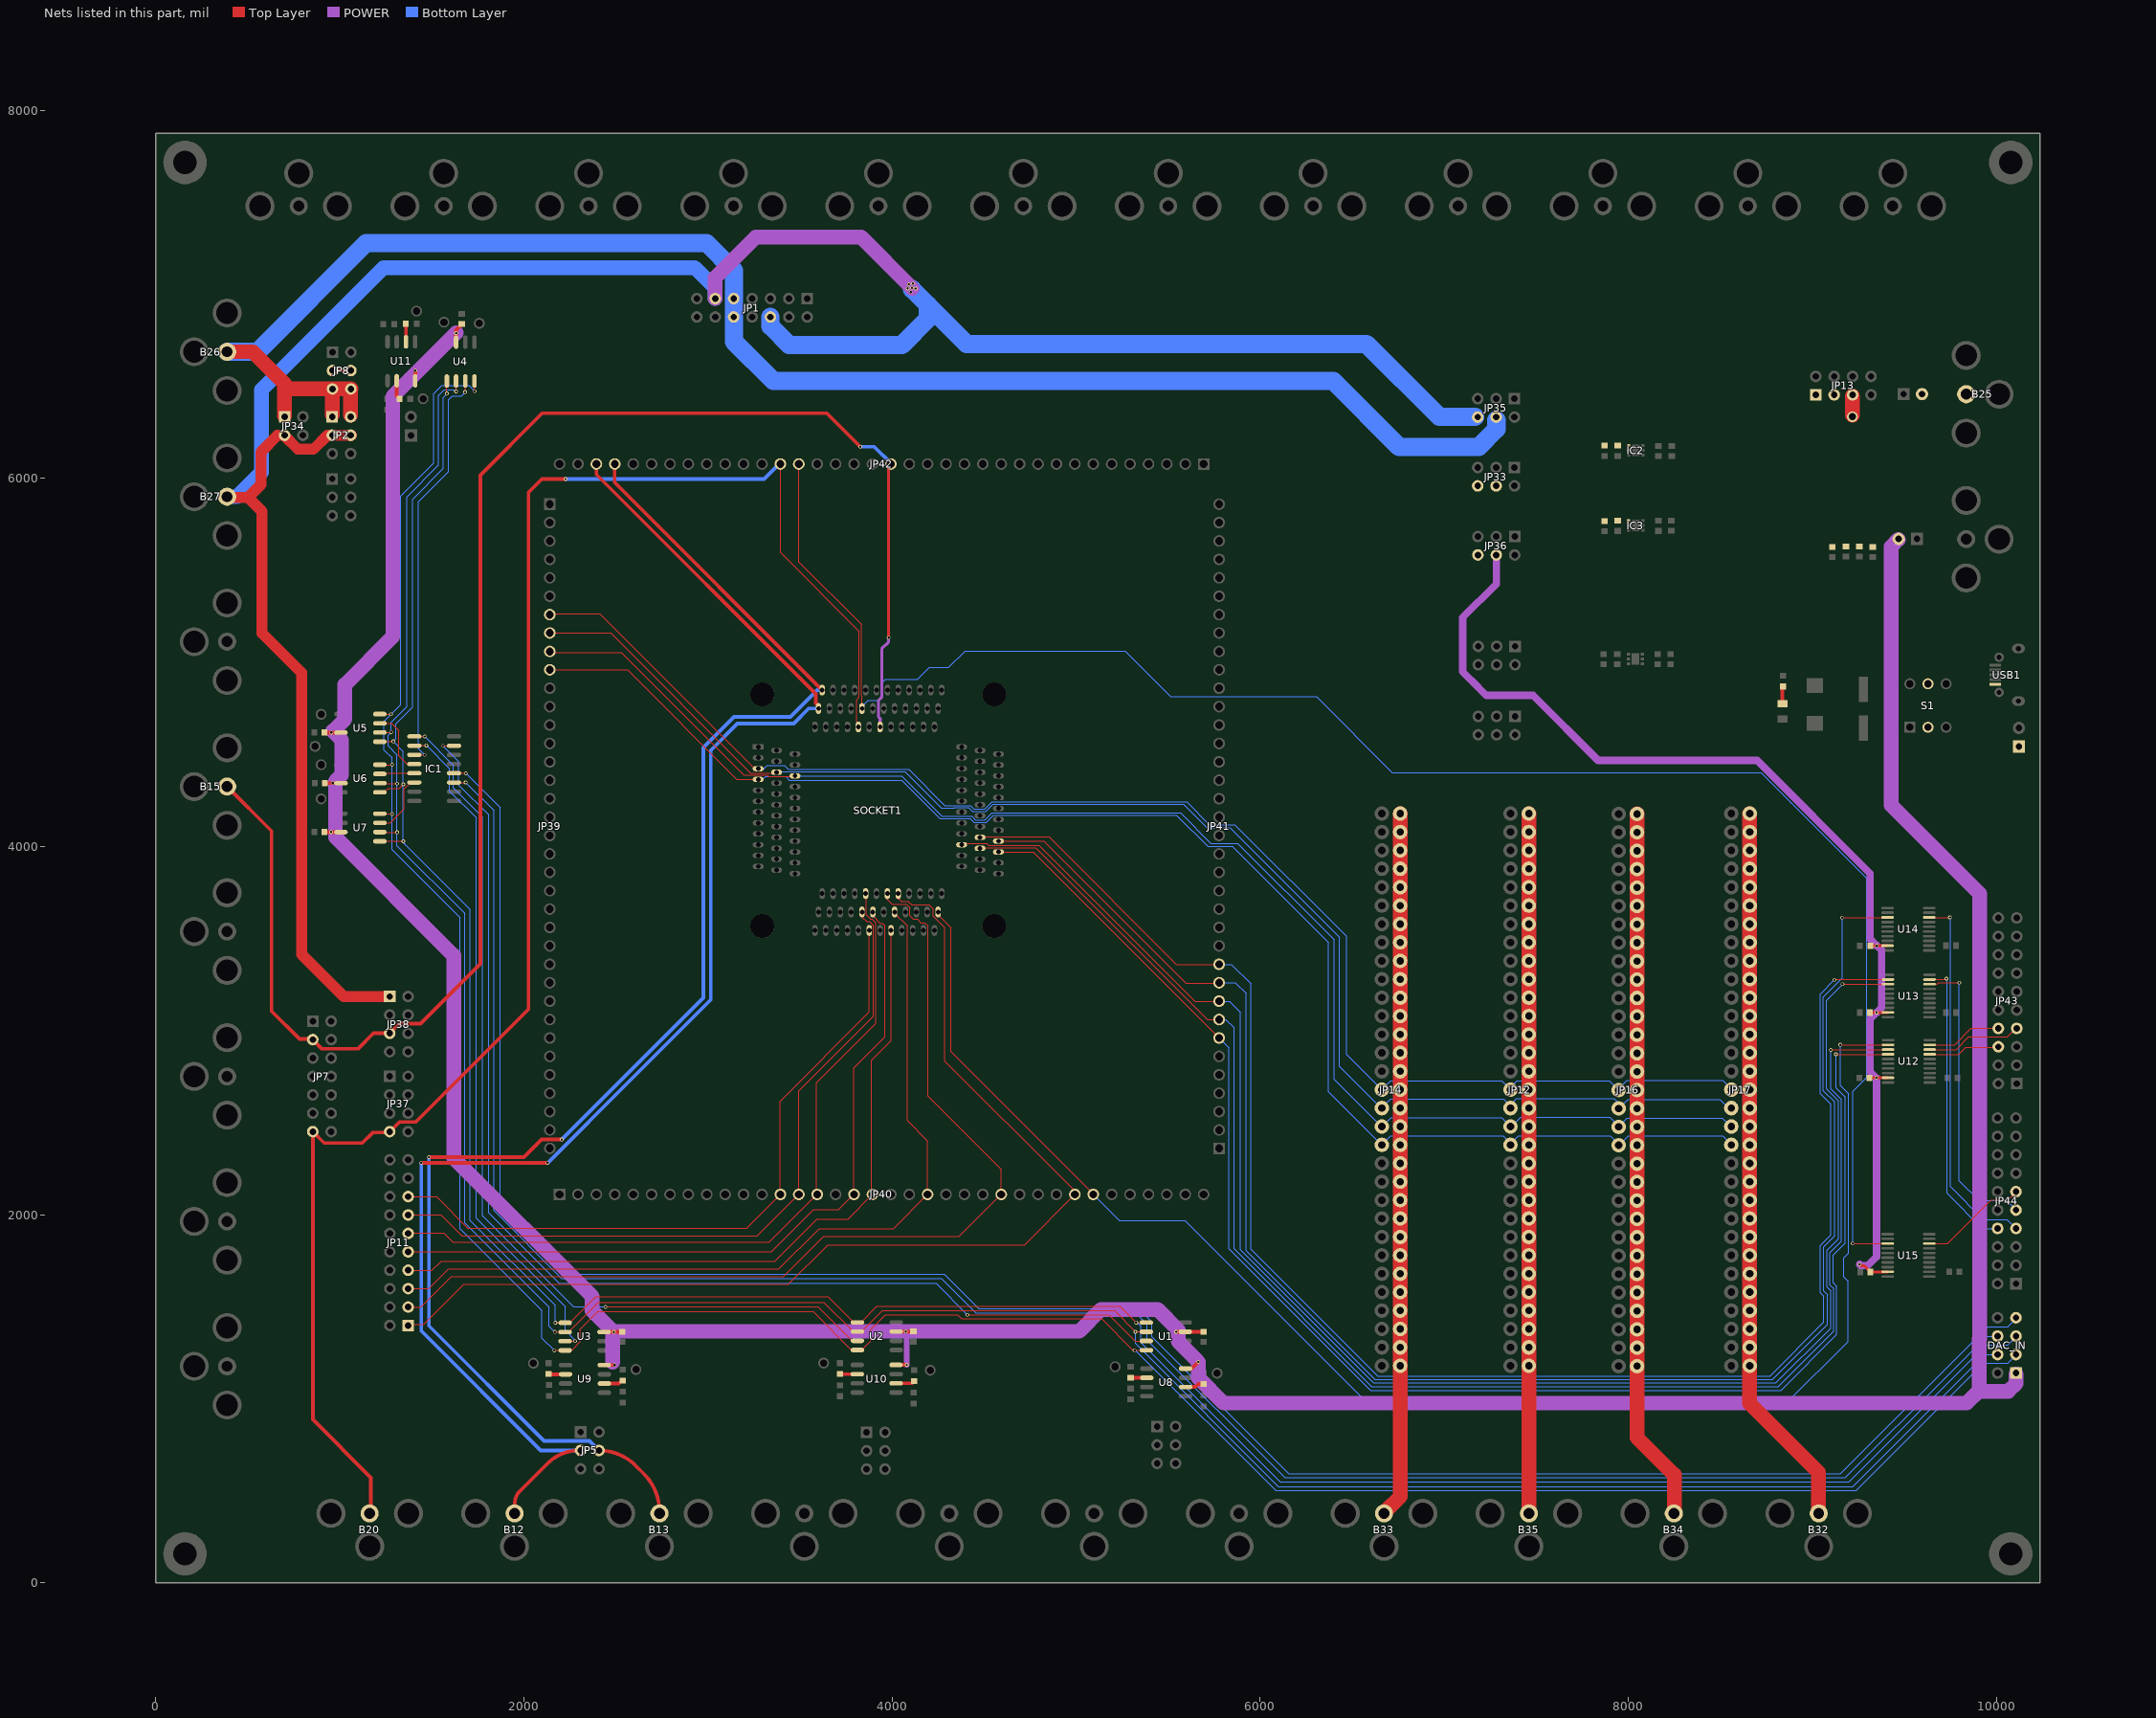
[diagram p0: the nets of this part, all layers, seen from the top]
# Altium PCB MISC62794.PcbDoc (part 4 of 7)
Units mil, origin at the board's own origin, x right, y up, seen from the top; angles counter-clockwise.
Board outline 10236.22 x 7874.02 mil, 4 copper layers (Top Layer, GND, POWER, Bottom Layer); 158 components, 185 nets, 1211 pads, 1759 vias.

## Via types
v1: diameter 20, hole 12, Top Layer to Bottom Layer, 1759 vias

## Nets (pads, with @x,y where several pads share a name; then routed paths per layer and width w, separated by ;. In a path a pad name is that pad's centre, name@x,y a point inside that pad or via, vN(x,y) a via of type N, cw(c..) or ccw(c..) an arc to the next point about the centre after c; other vN are vias at no path point) (continued)
IREF: B15.1 JP7.3 JP38.5 JP42.18 SOCKET1.126 | length 9370.4
  Top Layer w16: v1(3981,5135) 3981,6057 JP42.18@3993,6069
  Top Layer w20: B15.1@386.77,4325.69 628,4084.47 628,3106 780,2954 JP7.3@854,2954 ; JP7.3@852,2951 902,2901 1097,2901 1182,2986 ; 1222.43,2986 1182,2986 ; JP38.5@1258,2986 1182,2986 ; JP38.5@1269.93,2985.09 1321.83,3037 1437,3037 1762,3362 1762,5790 ; 1762,5819 1762,5790 ; v1(3827,6172) 3645,6354 2098,6354 1762,6018 1762,5790
  POWER w16: SOCKET1.126@3934.84,4649.77 3934.84,4695.16 3926.16,4703.84 3926.16,4793.16 3943.53,4810.53 3943.53,5074.53 3981,5112 v1(3981,5135)
  Bottom Layer w20: v1(3827,6172) 3903,6172 JP42.18@3988,6087
NetB25_1: B25.1 JP30.2
NetB32_1: B32.1 JP17.2 JP17.4 JP17.6 JP17.8 JP17.10 JP17.12 JP17.14 JP17.16 JP17.18 JP17.20 JP17.22 JP17.24 JP17.26 JP17.28 JP17.30 JP17.32 JP17.34 JP17.36 JP17.38 JP17.40 JP17.42 JP17.44 JP17.46 JP17.48 JP17.50 JP17.52 JP17.54 JP17.56 JP17.58 JP17.60 JP17.62 | length 3955.5
  Top Layer w80: JP17.62@8660,4179 JP17.60@8660,4079 JP17.58@8660,3979 JP17.56@8660,3879 JP17.54@8660,3779 JP17.52@8660,3679 JP17.50@8660,3579 JP17.48@8660,3479 JP17.46@8660,3379 JP17.44@8660,3279 JP17.42@8660,3179 JP17.40@8660,3079 JP17.38@8660,2979 JP17.36@8660,2879 JP17.34@8660,2779 JP17.32@8660,2679 JP17.30@8660,2579 JP17.28@8660,2479 JP17.26@8660,2379 JP17.24@8660,2279 JP17.22@8660,2179 JP17.20@8660,2079 JP17.18@8660,1979 JP17.16@8660,1879 JP17.14@8660,1779 JP17.12@8660,1679 JP17.10@8660,1579 JP17.8@8660,1479 JP17.6@8660,1379 JP17.4@8660,1279 JP17.2@8660,1179 8660,974 9033,601 B32.1@9033,378
NetB33_1: B33.1 JP14.2 JP14.4 JP14.6 JP14.8 JP14.10 JP14.12 JP14.14 JP14.16 JP14.18 JP14.20 JP14.22 JP14.24 JP14.26 JP14.28 JP14.30 JP14.32 JP14.34 JP14.36 JP14.38 JP14.40 JP14.42 JP14.44 JP14.46 JP14.48 JP14.50 JP14.52 JP14.54 JP14.56 JP14.58 JP14.60 JP14.62 | length 3836.9
  Top Layer w80: B33.1@6672.81,377.15 B33.1@6672.81,382 ; B33.1@6675,382 6762,469 6762,907 6762,1279 6762,1679 6762,2179 6762,2679 6762,3179 6762,3379 6762,3579 6762,3979 JP14.62@6762,4178
NetB34_1: B34.1 JP16.2 JP16.4 JP16.6 JP16.8 JP16.10 JP16.12 JP16.14 JP16.16 JP16.18 JP16.20 JP16.22 JP16.24 JP16.26 JP16.28 JP16.30 JP16.32 JP16.34 JP16.36 JP16.38 JP16.40 JP16.42 JP16.44 JP16.46 JP16.48 JP16.50 JP16.52 JP16.54 JP16.56 JP16.58 JP16.60 JP16.62 | length 3868.7
  Top Layer w80: JP16.62@8048,4177.02 JP16.60@8048,4077.02 JP16.58@8048,3977.02 JP16.56@8048,3877.02 JP16.54@8048,3777.02 JP16.52@8048,3677.02 JP16.50@8048,3577.02 JP16.48@8048,3477.02 JP16.46@8048,3377.02 JP16.44@8048,3277.02 JP16.42@8048,3177.02 JP16.40@8048,3077.02 JP16.38@8048,2977.02 JP16.36@8048,2877.02 JP16.34@8048,2777.02 JP16.32@8048,2677.02 JP16.30@8048,2577.02 JP16.28@8048,2477.02 JP16.26@8048,2377.02 JP16.24@8048,2277.02 JP16.22@8048,2177.02 JP16.20@8048,2077.02 JP16.18@8048,1977.02 JP16.16@8048,1877.02 JP16.14@8048,1777.02 JP16.12@8048,1677.02 JP16.10@8048,1577.02 JP16.8@8048,1477.02 JP16.6@8048,1377.02 JP16.4@8048,1277.02 JP16.2@8048,1177.02 8048,789 8250,587 B34.1@8250,392
NetB35_1: B35.1 JP12.2 JP12.4 JP12.6 JP12.8 JP12.10 JP12.12 JP12.14 JP12.16 JP12.18 JP12.20 JP12.22 JP12.24 JP12.26 JP12.28 JP12.30 JP12.32 JP12.34 JP12.36 JP12.38 JP12.40 JP12.42 JP12.44 JP12.46 JP12.48 JP12.50 JP12.52 JP12.54 JP12.56 JP12.58 JP12.60 JP12.62 | length 3786
  Top Layer w80: B35.1@7460,393 JP12.2@7460,1179 JP12.4@7460,1279 JP12.6@7460,1379 JP12.8@7460,1479 JP12.10@7460,1579 JP12.12@7460,1679 JP12.14@7460,1779 JP12.16@7460,1879 JP12.18@7460,1979 JP12.20@7460,2079 JP12.22@7460,2179 JP12.24@7460,2279 JP12.26@7460,2379 JP12.28@7460,2479 JP12.30@7460,2579 JP12.32@7460,2679 JP12.34@7460,2779 JP12.36@7460,2879 JP12.38@7460,2979 JP12.40@7460,3079 JP12.42@7460,3179 JP12.44@7460,3279 JP12.46@7460,3379 JP12.48@7460,3479 JP12.50@7460,3579 JP12.52@7460,3679 JP12.54@7460,3779 JP12.56@7460,3879 JP12.58@7460,3979 JP12.60@7460,4079 JP12.62@7460,4179
NetJP13_5: JP13.5 TP15.1 | length 104
  Top Layer w80: TP15.1@9218,6343 JP13.5@9218,6447
NetJP32_1: JP32.1 S1.2
NetLED_BLUE_2: LED_BLUE.2 R20.1 | length 82.7
  Top Layer w20: LED_BLUE.2@8838,4775.33 R20.1@8838,4858
NetR1_1: R1.1 U8.2 | length 80.8
  Top Layer w20: R1.1@5302.67,1113.67 U8.2@5383.51,1113.67
NetR3_2: R3.2 U8.6 | length 99
  Top Layer w20: U8.6@5594.73,1063.67 5648.67,1063.67 5665,1080 R3.2@5687,1080
NetR5_1: R5.1 U10.2 | length 90.2
  Top Layer w20: R5.1@3720.33,1133.67 U10.2@3810.51,1133.67
NetR7_2: R7.2 U10.6 | length 102.8
  Top Layer w20: U10.6@4021.73,1083.67 4105.67,1083.67 R7.2@4119,1097
NetR9_1: R9.1 U9.2 | length 88.2
  Top Layer w20: R9.1@2137.33,1132.67 U9.2@2225.51,1132.67
NetR11_2: R11.2 U9.6 | length 101
  Top Layer w20: U9.6@2436.73,1082.67 2514.67,1082.67 R11.2@2531,1099
NetR13_1: R13.1 U11.2 | length 86.3
  Top Layer w20: U11.2@1358.29,6741.99 R13.1@1358.29,6828.29
NetR15_2: R15.2 U11.6 | length 103.9
  Top Layer w20: U11.6@1308.29,6530.77 1308.29,6447.71 R15.2@1323,6433
NetS1_5: S1.5 USB1.1
OEN: JP41.9 SOCKET1.81 U13.13 | length 9034.7
  Top Layer w6: SOCKET1.81@4385,4009 4393,4017 4515,4017 4525.68,4006.32 4798.68,4006.32 5644.98,3160.02 JP41.9@5777,3160.02 ; v1@9168.01,3251.99 U13.13@9410.97,3251.99
  Bottom Layer w6: JP41.9@5777,3160.02 5831.98,3160.02 5893,3099 5893,1976 ; 5893,1960 5893,1976 ; v1@9163,3250 9078,3165 9078,2893 9078,2683 9142,2619 9142,1869 9081,1808 9081,1606 9101,1586 9101,1384 8803,1086 6616,1086 5893,1809 5893,1976 ; v1@9164,3250 v1(9164,3252)
OEN_MCU: JP44.9 U13.8 | length 1615.6
  Top Layer w6: U13.8@9637.03,3251.99 9678.99,3251.99 9687,3260 v1(9799,3260)
  Bottom Layer w6: v1@9804,3259 9799,3254 9799,2185 9907,2077 10055.01,2077 JP44.9@10107,2025.01
OUT<0>: JP11.1 JP40.29 SOCKET1.60 | length 6042.2
  Top Layer w6: JP11.1@1384,1404 1455,1404 1673,1622 3437,1622 3651,1836 4718.98,1836 JP40.29@4993,2110.02 ; SOCKET1.60@4033.27,3744.26 4033.27,3718.73 4049,3703 4086,3703 4106.21,3682.79 4200.43,3682.79 4223,3660.22 4223,3622 4287,3558 4287,2835 4947,2175 ; 4970,2152 4947,2175 ; JP40.29@5004,2115 5004,2118 4947,2175
OUT<1>: JP11.5 JP40.21 SOCKET1.59 | length 4653
  Top Layer w6: JP11.5@1370.64,1598.09 1482.09,1598.09 1589,1705 3384,1705 3604,1925 4007.98,1925 JP40.21@4193,2110.02 ; SOCKET1.59@4013.58,3644.26 4013.58,3638.42 4082,3570 4082,2511 4193,2400 4193,2186 ; JP40.21@4193,2124 4193,2186 ; 4193,2162 4193,2186
OUT<2>: JP11.7 JP40.18 SOCKET1.58 | length 4134.8
  Top Layer w6: JP11.7@1388,1697 1500,1697 1551,1748 3363,1748 3592,1977 3759.98,1977 JP40.18@3893,2110.02 ; JP40.18@3889,2129 3889,2840 3993.9,2944.9 SOCKET1.58@3993.9,3544.26
OUT<3>: JP11.3 JP40.25 SOCKET1.57 | length 5460.1
  Top Layer w6: JP11.3@1370.64,1498.09 1440.09,1498.09 1605,1663 3410,1663 3628,1881 4363.98,1881 JP40.25@4593,2110.02 ; SOCKET1.57@3974.21,3744.26 3974.21,3712.79 3999.95,3687.05 4078.05,3687.05 4096.01,3669.1 4096.01,3623.99 4115,3605 4138,3605 4157,3586 4177.53,3586 4194.43,3569.1 4194.43,2644.57 4594,2245 4594,2204 ; JP40.25@4594,2127 4594,2204 ; 4594,2165 4594,2204
OUT<4>: JP11.9 JP40.17 SOCKET1.53 | length 4217.7
  Top Layer w6: JP11.9@1374,1799 1473,1799 ; 1421,1799 1473,1799 ; JP40.17@3793,2110.02 3709.98,2027 3573,2027 3345,1799 1473,1799 ; JP40.17@3793,2127 3793,2189 ; 3793,2180 3793,2189 ; SOCKET1.53@3895.47,3636.53 SOCKET1.53@3895.47,3644.26 ; SOCKET1.53@3898,3624 3898,3621 3936.21,3582.79 3949.21,3582.79 3962,3570 3962,2967 3793,2798 3793,2189
OUT<5>: JP11.15 JP40.13 SOCKET1.52 | length 3798.7
  Top Layer w6: JP11.15@1380,2098 1524,2098 1695,1927 3209.98,1927 JP40.13@3393,2110.02 ; JP40.13@3391,2124 3391,2180 ; 3391,2162 3391,2180 ; SOCKET1.52@3875.79,3544.26 3875.79,3100.79 3391,2616 3391,2180
OUT<6>: JP11.11 JP40.15 SOCKET1.51 | length 4130.2
  Top Layer w6: JP11.11@1375,1900 1564,1900 1614,1850 3332.98,1850 JP40.15@3593,2110.02 ; JP40.15@3590,2139 3590,2192 ; 3590,2174 3590,2192 ; SOCKET1.51@3856.1,3744.26 3859.79,3740.57 3859.79,3629.21 3883.27,3605.73 3891.27,3605.73 3911.16,3585.84 3911.16,3038.16 3590,2717 3590,2192
OUT<7>: JP11.13 JP40.14 SOCKET1.50 | length 4007.3
  Top Layer w6: JP11.13@1375,2000 1548,2000 1663,1885 3267.98,1885 JP40.14@3493,2110.02 ; JP40.14@3493,2120 3493,2202 ; 3493,2182 3493,2202 ; SOCKET1.50@3836.42,3644.26 3836.42,3616.58 3861,3592 3878,3592 3899.16,3570.84 3899.16,3079.16 3493,2673 3493,2202
RCLK: DAC_IN.7 IC1.12 | length 11719.8
  Top Layer w6: IC1.12@1619.33,4398.08 v1(1683.08,4398.08)
  Bottom Layer w6: v1(1683.08,4398.08) 1870,4211.16 1870,2024 2218,1676 4284,1676 4470,1490 5341,1490 5413,1418 5413,1335 6155,593 9154,593 9953,1392 10064,1392 DAC_IN.7@10091,1419
READ_EN: JP41.11 SOCKET1.83 U13.12 | length 8978.2
  Top Layer w6: SOCKET1.83@4498.94,4053.06 4851.94,4053.06 5544.98,3360.02 JP41.11@5777,3360.02 ; v1@9124,3274 9127.58,3277.58 U13.12@9410.97,3277.58
  Bottom Layer w6: JP41.11@5777,3360.02 5842.98,3360.02 5949,3254 5949,1813 6639,1123 8770,1123 9063,1416 9063,1558 9045,1576 9045,1834 9101,1890 9101,2599 9043,2657 9043,3199 v1@9120,3276
  other v1: 9121,3276
READ_EN_MCU: JP44.8 U13.9 | length 1612.5
  Top Layer w6: U13.9@9637.03,3277.58 9724.58,3277.58 v1(9729,3282)
  Bottom Layer w6: v1@9732,3280 9732,2115 9921.99,1925.01 JP44.8@10007,1925.01
SCLK: DAC_IN.6 IC1.11 | length 11592.8
  Top Layer w6: IC1.11@1619.33,4348.08 v1(1682.92,4348.08)
  Bottom Layer w6: v1(1682.92,4348.08) 1836,4195 1836,2022 2204,1654 4269,1654 4455.5,1467.5 5323.5,1467.5 5387,1404 5387,1318 6134,571 9179,571 9742,1134 ; 9745,1137 9742,1134 ; 9966.5,1340 9958,1340 ; DAC_IN.6@9993,1340 9958,1340 ; 9742,1134 9948,1340 9958,1340
SPI_CLK: DAC_IN.5 U1.1 U2.1 U3.1 U4.1 U5.1 U6.1 U7.1 | length 14765.3
  Top Layer w6: U7.1@1216.15,4028.46 v1(1344.54,4028.46) ; U5.1@1235,4571 v1(1290,4571) ; U6.1@1247,4301 1262,4316 1322,4316 v1(1344,4338) ; v1(1580.71,6461.29) U4.1@1580.71,6529.01 ; v1(2170.33,1412.67) U3.1@2223.51,1412.67 ; U3.1@2245,1410 2390,1555 3652,1555 3792.33,1414.67 U2.1@3811.51,1414.67 ; U2.1@3835,1420 3918,1503 5237.34,1503 v1(5326.67,1413.67) U1.1@5381.51,1413.67
  Bottom Layer w6: 1352,4013 1356,4009 ; v1@1578.5,6457.5 v1@1581,6460 ; v1@1579,6457 1562,6440 1562,6054 1395,5887 1395,4757 1305,4667 1305,4586 v1(1290,4571) 1344,4517 v1(1344,4338) 1344,4021 1356,4009 ; v1(2170.33,1412.67) 2170.33,1506.67 1708,1969 1708,3657 1356,4009 ; v1(5326.67,1413.67) 5330.33,1413.67 5351,1393 5351,1306 6109,548 9200,548 9777,1125 ; 9779,1127 9777,1125 ; DAC_IN.5@10099,1329 10062,1292 9944,1292 9777,1125
SPI_CS1: IC1.15 U1.3 | length 6545.5
  Top Layer w6: v1(1559,4547) 1599,4547 IC1.15@1600,4546 ; v1(4409,1456) 4409,1457 5177,1457 5320.33,1313.67 U1.3@5381.51,1313.67
  Bottom Layer w6: v1(1559,4547) 1645,4461 1645,4335 1807,4173 1807,2010 2190,1627 4238,1627 v1(4409,1456)
SPI_CS2: IC1.1 U2.3 | length 5080.4
  Top Layer w6: IC1.1@1434,4599 1435,4598 v1(1460,4598) ; v1(2443,1499) 3597,1499 3781.33,1314.67 U2.3@3811.51,1314.67
  Bottom Layer w6: v1(1460,4598) 1617,4441 1617,4319 1775,4161 1775,1993 2268,1500 v1@2442,1500 ; v1(2443,1499) v1@2442,1500 ; v1@2443,1500 v1@2442,1500
SPI_CS3: IC1.2 U3.3 | length 3676.6
  Top Layer w6: IC1.2@1421,4552 1424,4549 v1(1469,4549) ; U3.3@2223.51,1312.67 v1(2277.33,1312.67)
  Bottom Layer w6: v1(1469,4549) 1596,4422 1596,4300 1740,4156 1740,1982 2223,1499 2223,1372 v1@2277.33,1317.67 ; v1(2277.33,1312.67) v1@2277.33,1317.67 ; v1@2279,1316 v1@2277.33,1317.67
SPI_CS4: IC1.3 U4.3 | length 2220.9
  Top Layer w6: IC1.3@1403.94,4498.08 v1(1459.92,4498.08) ; v1(1680,6469) U4.3@1680,6508
  Bottom Layer w6: v1(1459.92,4498.08) 1426,4532 1426,5874 1590,6038 1590,6293 ; 1590,6300 1590,6293 ; v1@1677,6466 v1(1680,6469) ; v1@1678,6465 1661,6448 1611,6448 1590,6427 1590,6379 1590,6376 1590,6293
SPI_CS5: IC1.4 U5.3 | length 339.3
  Top Layer w6: U5.3@1238,4670 1280,4670 1319,4631 1319,4492 1362.92,4448.08 IC1.4@1403.94,4448.08
SPI_CS6: IC1.5 U6.3 | length 153.9
  Top Layer w6: U6.3@1250.08,4398.08 IC1.5@1403.94,4398.08
SPI_CS7: IC1.6 U7.3 | length 342
  Top Layer w6: U7.3@1216.15,4128.46 1272.46,4128.46 1348,4204 1348,4312 1384.08,4348.08 IC1.6@1403.94,4348.08
SPI_MISO: DAC_IN.3 U1.4 U2.4 U3.4 U4.4 U5.4 U6.4 U7.4 | length 15066.1
  Top Layer w6: U7.4@1237,4178 1238,4177 v1(1283,4177) ; U5.4@1241,4718 v1@1276,4718 ; U6.4@1243,4446 1245,4444 v1(1283,4444) ; v1(1731,6474) U4.4@1731,6503 ; v1(2164.67,1262.67) U3.4@2223.51,1262.67 ; U3.4@2236,1265 2262,1265 2306,1309 2306,1378 2402,1474 3570,1474 3779.33,1264.67 U2.4@3811.51,1264.67 ; U2.4@3836,1267 3837,1267 3884,1314 3884,1375 3964,1455 4355,1455 4376,1434 5138,1434 5308.33,1263.67 v1(5317.67,1263.67) U1.4@5381.51,1263.67
  Bottom Layer w6: v1(1731,6474) 1701,6504 1554,6504 1510,6460 1510,6084 1330,5904 1330,4772 v1(1277,4719) 1239,4681 1239,4525 1283,4481 v1(1283,4444) v1(1283,4177) 1283,3984 1652,3615 1652,1925 2098,1479 2098,1329.34 v1(2164.67,1262.67) ; v1@5321.33,1263.67 6084,501 9239,501 9930,1192 10062,1192 DAC_IN.3@10091,1221
SPI_MOSI: DAC_IN.4 U1.2 U2.2 U3.2 U4.2 U5.2 U6.2 U7.2 | length 14708.1
  Top Layer w6: U5.2@1216.15,4619.46 1279.46,4619.46 v1@1281,4621 ; U7.2@1233,4079 1235,4077 v1(1310,4077) ; U6.2@1235,4342 v1(1310,4342) ; U4.2@1630,6501 1631,6500 v1(1631,6472) ; v1(2166.67,1362.67) U3.2@2223.51,1362.67 2241.67,1362.67 2403,1524 3629,1524 U2.2@3789,1364 ; U2.2@3811.51,1364.67 3833.67,1364.67 3947,1478 5208,1478 v1@5318,1368 ; v1(5322.33,1363.67) U1.2@5381.51,1363.67
  Bottom Layer w6: 1536,6296 1536,6291 ; v1@1627,6474 1619,6482 1567,6482 1536,6451 1536,6291 ; v1@1628,6475 v1(1631,6472) ; v1(2166.67,1362.67) 2136,1393.34 2136,1497 1678,1955 1678,3637 1310,4005 v1(1310,4077) v1(1310,4342) 1310,4497 1261,4546 1261,4605 v1(1278,4622) 1278,4675 1363,4760 1363,5899 1536,6072 1536,6291 ; v1(5322.33,1363.67) 5322.33,1299.67 6099,523 9221,523 9804,1106 ; 9809,1111 9804,1106 ; DAC_IN.4@9986,1239 9937,1239 9804,1106
STATE<0>: JP41.7 SOCKET1.79 U12.14 | length 8514.4
  Top Layer w6: SOCKET1.79@4580,3969 4768.02,3969 JP41.7@5777,2960.02 ; v1(9128.6,2871.4) U12.14@9411.97,2871.4
  Bottom Layer w6: JP41.7@5777,2960.02 5830,2907.02 5830,2096 ; 5830,1970 5830,2096 ; v1@9129,2869 9129,2689 9134,2684 9178,2640 9178,1847 9113,1782 9113,1629 9133,1609 9133,1348 8831,1046 6599,1046 5830,1815 5830,2096
STATE<0>_MCU: JP43.6 U12.7 | length 376
  Top Layer w6: U12.7@9638.03,2871.4 9794.4,2871.4 9833,2910 JP43.6@9998,2910
STATE<1>: JP41.8 SOCKET1.80 U12.13 | length 8566.2
  Top Layer w6: SOCKET1.80@4477.76,3990.32 4481.44,3994.01 4778.99,3994.01 5714,3059 JP41.8@5766,3059 ; v1@9102,2900 9105.01,2896.99 U12.13@9411.97,2896.99
  Bottom Layer w6: JP41.8@5777,3060.02 5812.98,3060.02 5858,3015 5858,1814 6605,1067 8816,1067 9117,1368 9117,1598 9097,1618 9097,1794 9158,1855 9158,2627 9101,2684 v1(9101,2895)
STATE<1>_MCU: JP43.7 U12.8 | length 504.3
  Top Layer w6: U12.8@9638.03,2896.99 9781.99,2896.99 9851,2966 10060,2966 JP43.7@10098,3004
STATE<2>: JP40.30 SOCKET1.71 U12.12 | length 8549.5
  Top Layer w6: SOCKET1.71@4249.8,3644.26 4249.8,3628.2 4319,3559 4319,2887 5027.5,2178.5 ; 5064,2142 5027.5,2178.5 ; JP40.30@5096,2117 5089,2117 5027.5,2178.5 ; v1(9152.42,2922.58) U12.12@9411.97,2922.58
  Bottom Layer w6: JP40.30@5093,2110.02 5235.02,1968 5590,1968 6579,979 8862,979 9194,1311 9194,1639 9174,1659 9172.01,1660.99 9172.01,1764.01 9198,1790 9198,2657 9153,2702 v1@9153,2922
STATE<2>_MCU: JP43.8 U12.9 | length 415
  Top Layer w6: U12.9@9638.03,2922.58 9774.58,2922.58 9864,3012 JP43.8@10016,3012
STROBE: JP41.10 SOCKET1.82 U14.13 | length 9228.7
  Top Layer w6: SOCKET1.82@4577.76,4029.69 4824.31,4029.69 5596,3258 JP41.10@5766,3258 ; v1@9166.01,3614.99 U14.13@9408.97,3614.99
  Bottom Layer w6: JP41.10@5777,3260.02 5864.98,3260.02 5923,3202 5923,1986 ; 5923,1960 5923,1986 ; v1(9163,3614) 9163,3286 9060,3183 9060,2673 9121,2612 9121,1884 9063,1826 9063,1587 9084,1566 9084,1405 8784,1105 6623,1105 5923,1805 5923,1986
STROBE_MCU: JP44.7 U14.8 | length 2027
  Top Layer w6: U14.8@9635.03,3614.99 v1(9748.01,3614.99)
  Bottom Layer w6: v1@9751,3616 9751,2152 9929,1974 10058.01,1974 JP44.7@10107,1925.01
TEST_PS_CTRL: B20.1 JP7.13 JP37.7 JP42.24 SOCKET1.132 | length 9493.8
  Top Layer w6: JP42.24@3393,6078.02 3393,5597 3820.42,5169.58 3820.42,4811.42 3807,4798 3807,4677 SOCKET1.132@3817,4667
  Top Layer w20: B20.1@1168,417 1168,571 852,887 JP7.13@852,2451 914,2389 1121,2389 1178,2446 JP37.7@1255,2446 ; JP37.7@1269.93,2451.09 1322.43,2503.6 1412.6,2503.6 2024,3115 2024,5817 ; 2024,5827 2024,5817 ; v1(2226,5997) 2097,5997 2024,5924 2024,5817
  Bottom Layer w20: v1(2226,5997) 2294,5997 3305,5997 JP42.24@3380,6072 ; JP42.24@3383.49,6068.51 JP42.24@3393,6078.02
TESTDELAY_IN: JP42.23 SOCKET1.131 U15.13 | length 9791.4
  Top Layer w6: JP42.23@3494,6064 3494,5545 3832.42,5206.58 3832.42,4822 3836.42,4818 SOCKET1.131@3836.42,4749.77 ; v1@9222.01,1842.99 U15.13@9409.97,1842.99
  Bottom Layer w6: SOCKET1.131@3846,4770 3852.5,4776.5 3870,4794 3922,4794 3945,4817 3945,4889 3964,4908 4138,4908 4203,4973 4307,4973 4397,5063 5265,5063 5514,4814 6305,4814 6718,4401 8721,4401 8877.5,4244.5 ; 8883,4239 8877.5,4244.5 ; v1(9220,1843) 9220,2670 9295,2745 9295,3827 8877.5,4244.5
TESTDELAY_IN_MCU: JP44.11 U15.8 | length 566.7
  Top Layer w6: U15.8@9636.03,1842.99 9734.99,1842.99 9971,2079 10064,2079 JP44.11@10093,2108
USB_5V: C1.2 C2.2 C3.2 C4.2 C5.2 C6.2 C7.2 C8.1 C9.1 C10.1 C11.1 DAC_IN.1 JP13.1 JP13.3 JP31.2 U1.7 U2.7 U3.7 U4.7 U5.7 U6.7 U7.7 U8.8 U9.8 U10.8 U11.8 | length 20564.8
  Top Layer w20: C5.2@919.54,4619.46 v1@951,4619.46 ; C7.2@920,4083 924.54,4078.46 v1@951,4078.46 ; C6.2@927.54,4344.46 v1@965,4344.46 ; v1(951.46,4078.46) v1@951,4078.46 ; v1(952.54,4619.46) U5.7@1004.93,4619.46 ; v1(960.46,4344.46) v1@965,4344.46 ; U7.7@1004.93,4078.46 v1@951,4078.46 ; U6.7@1004.93,4344.46 v1@965,4344.46 ; U11.8@1408.29,6530.77 v1(1408.29,6585.71) ; U4.7@1630.71,6740.23 v1@1630.71,6790 ; v1(1631,6790) v1@1630.71,6790 ; C4.2@1656,6832 1630.71,6806.71 v1@1630.71,6790 ; U3.7@2434.73,1362.67 C3.2@2534.12,1362.67 ; U9.8@2436.73,1182.67 v1(2491.67,1182.67) ; U10.8@4021.73,1183.67 v1(4079.33,1183.67) ; U2.7@4022.73,1364.67 C2.2@4110.33,1364.67 ; v1(5543.67,1363.67) U1.7@5592.73,1363.67 C1.2@5684.67,1363.67 ; U8.8@5594.73,1163.67 5627.67,1163.67 v1(5664,1200)
  POWER w30: v1(4079.33,1183.67) 4079.33,1331.67
  POWER w80: v1(1631,6790) 1287,6446 1287,5140 1026,4879 1026,4692 961,4627 1009,4579 1009,4389 975,4355 975,4051 1618,3408 1618,2307 2370,1555 2370,1478 v1@2482,1366 ; 2482,1199 v1@2482,1366 ; 3914,1366 3867,1366 ; 5655,1211 5554,1312 5554,1374 5443,1485 5136,1485 5017,1366 3867,1366 ; v1(5664,1200) 5664,1113 5801,976 9839,976 9907,1044 ; JP31.2@9467,5668 9429,5630 9429,4224 9909,3744 9909,1327 9907,1325 9907,1044 ; 9913,1050 9907,1044 ; DAC_IN.1@10108,1133 10108,1083 10065,1040 9907,1040 9907,1044 ; v1@2482,1366 3867,1366
  other v1: 2488,1363 4074,1365
V11: B27.1 C21.1 C22.1 IC2.1 JP1.6 JP1.11 JP2.3 JP2.4 JP33.6 JP34.3 JP35.6 JP36.6 JP38.1 | length 13512.6
  Top Layer w50: JP2.4@1057.64,6235 JP2.4@1059,6235
  Top Layer w60: B27.1@394,5897 500,5897 ; JP2.4@1061,6235 1057.64,6235 932,6235 855,6158 772,6158 696,6234 660,6234 570,6144 570,5967 500,5897 ; JP38.1@1269.93,3185.09 1019.91,3185.09 791,3414 791,4944 576,5159 576,5821 500,5897
  POWER w80: JP1.11@3039,6977 3039,7090 3260,7311 3831,7311 4110,7032 v1@4109,7032
  Bottom Layer w80: B27.1@386.77,5900.5 440.5,5900.5 573,6033 573,6481 1237,7145 2927,7145 3039,7033 JP1.11@3039,6977 ; JP35.6@7167,6332 JP35.6@7176,6332
  Bottom Layer w100: JP1.6@3339,6877 3339,6827 3441,6725 4053,6725 4195,6867 4195,6942 v1@4109,7028 ; 4195,6940 4405,6730 6578,6730 6974,6334 JP35.6@7167,6334
  other v1: 4101,7012 4128,7031 4084,7032 4108,7035 4091,7055 4113,7059
V25: B26.1 C25.1 C26.1 C30.2 C32.2 C34.2 C36.2 IC3.1 JP1.9 JP1.10 JP2.1 JP2.2 JP8.5 JP8.6 JP33.4 JP34.1 JP35.4 JP36.4 U12.19 U13.19 U14.19 U15.19 | length 15230.5
  Top Layer w16: v1(9257,1730) 9265,1722 9282.57,1722 C36.2@9315.56,1689.01 ; C30.2@9310.99,2743.44 U12.19@9411.97,2743.44 ; C32.2@9312.99,3098.44 v1(9349.44,3098.44) ; C34.2@9315.99,3461.44 v1@9350,3461.44 ; C36.2@9323.44,1689.44 U15.19@9409.97,1689.44 ; v1@9350.44,3461.44 U14.19@9408.97,3461.44 ; v1@9351,3098.44 U13.19@9410.97,3098.44
  Top Layer w80: B26.1@386.77,6687.9 526.1,6687.9 699,6515 JP34.1@699,6340 ; 727.98,6486.02 JP8.5@959,6486.02 JP8.6@1059,6486.02 ; JP2.1@957.64,6345 JP8.5@957.64,6484.65 ; JP2.2@1057.64,6344 JP8.6@1057.64,6484.65
  POWER w40: 7183,4867 7229,4821 7483,4821 7836,4468 8700,4468 9315,3853 9315,3498 v1@9349,3464 ; 7183.5,4867.5 7100,4951 7100,5243 7283,5426 JP36.4@7283,5569 ; JP36.4@7281,5569 JP36.4@7281,5576 ; v1(9257,1730) 9264,1723 9301,1723 9349,1771 9349,2742 9314,2777 9314,3062 9349,3097 v1@9349,3098.44 ; v1@9349,3461 v1@9349,3464 ; v1@9350,3098 9377,3125 9377,3436 v1@9349,3464
  Bottom Layer w80: 7282,6273 JP35.4@7282,6328
  Bottom Layer w100: B26.1@386.77,6687.9 551.9,6687.9 1143,7279 2991,7279 3141,7129 3141,6743 3355,6529 6397,6529 6755,6171 7187,6171 7284,6268 JP35.4@7284,6317
  other v1: 9348,2744 9350.44,3461
VBIT1: B12.1 JP5.3 JP42.34 SOCKET1.143 | length 8394.4
  Top Layer w6: SOCKET1.143@3600.2,4749.77 SOCKET1.143@3600.2,4766
  Top Layer w20: v1(1442,2282) v1(2128,2282) ; B12.1@1948.4,377.15 B12.1@1948.4,382 ; B12.1@1949,382 1949,428.58 cw(c2049,428.58) 1978.29,499.29 2128,649 ; 2131,652 2128,649 ; JP5.3@2307.19,719.02 2297.03,719.02 ccw(c2297.03,479.97) 2128,649 ; JP42.34@2393,6078.02 2393,6021 3585,4829 3585,4780 SOCKET1.143@3599,4766
  Bottom Layer w20: v1(1442,2282) 1442,1368 2090.98,719.02 JP5.3@2307.19,719.02 ; v1(2128,2282) 2129.15,2282 2352,2504.85 2352,2506 3015,3169 3015,4524 3159,4668 3465,4668 3546.77,4749.77 SOCKET1.143@3600.2,4749.77
VBIT2: B13.1 JP5.4 JP42.33 SOCKET1.142 | length 8305.7
  Top Layer w20: v1(1483,2312) 1999,2312 2095,2408 v1(2205,2408) ; JP5.4@2407.19,719.02 cw(c2407.19,437.05) 2606.57,636.43 2650.44,592.56 cw(c2443.88,386) B13.1@2736,386 ; JP42.33@2492,6070 2492,5977.65 SOCKET1.142@3619.88,4849.77
  Bottom Layer w20: v1(1483,2312) 1483,1396 2109,770 2356.2,770 JP5.4@2407.19,719.02 ; v1(2205,2408) 2975,3178 2975,4538 3141,4704 3448,4704 3593.77,4849.77 SOCKET1.142@3619.88,4849.77
VBIT_FORMING: JP8.3 JP8.4 | length 102
  Top Layer w20: JP8.3@959,6586.02 JP8.4@1059,6586.02 JP8.4@1060.98,6586.02
VBIT_FORMING<0>: JP12.31 JP14.31 JP16.31 JP17.31 JP39.7 SOCKET1.7 | length 7984.4
  Top Layer w6: JP39.7@2159,5265 2412,5265 3253.61,4423.39 SOCKET1.7@3272.24,4423.39
  Bottom Layer w6: SOCKET1.7@3272.24,4423.39 3304.39,4423.39 3320.39,4439.39 3415.61,4439.39 3435.29,4419.71 4090.29,4419.71 4287.14,4222.86 4402.59,4222.86 4402.74,4223 4426,4223 4445.83,4203.17 4504.17,4203.17 4543.54,4242.54 5601.46,4242.54 5725,4119 5862,4119 6469,3512 6469,2870 JP14.31@6639,2700 ; JP14.31@6661,2679 6709.37,2727.37 7311.63,2727.37 7354,2685 7396.37,2727.37 7897.63,2727.37 7945,2680 7993.65,2728.65 8514.35,2728.65 JP17.31@8565,2678
VBIT_FORMING<1>: JP12.29 JP14.29 JP16.29 JP17.29 JP39.8 SOCKET1.8 | length 7977.9
  Top Layer w6: JP39.8@2140,5160.02 2470.98,5160.02 3230.98,4400.02 3354.02,4400.02 SOCKET1.8@3355,4401
  Bottom Layer w6: SOCKET1.8@3372.24,4403.71 3375.93,4407.39 4070.61,4407.39 4268,4210 4337,4210 4337.54,4210.54 4416.46,4210.54 4435.83,4191.17 4509.14,4191.17 4548.2,4230.23 5583.77,4230.23 5712,4102 5836,4102 6432,3506 6432,2804 JP14.29@6640,2596 ; JP14.29@6661,2579 6709.37,2627.37 7321.63,2627.37 7356,2593 7393,2630 7922,2630 7962,2590 7998,2626 8499,2626 JP17.29@8545,2580
VBIT_FORMING<2>: JP12.27 JP14.27 JP16.27 JP17.27 JP39.9 SOCKET1.9 | length 8030.2
  Top Layer w6: JP39.9@2144,5054 2528,5054 3193.98,4388.02 3321,4388.02 3328.69,4380.34 3468.56,4380.34 SOCKET1.9@3472.24,4384.02
  Bottom Layer w6: SOCKET1.9@3472.24,4384.02 4050.98,4384.02 4271.2,4163.8 4433.23,4163.8 4452.92,4144.12 4504.12,4144.12 4543.49,4183.49 5566.51,4183.49 5732,4018 5877,4018 6402,3493 6402,2736 JP14.27@6644,2494 ; JP14.27@6661,2479 6664.26,2479 6712.63,2527.37 7312.63,2527.37 7342,2498 7386,2498 7417,2529 7899,2529 7941,2487 7954,2487 7992.39,2525.39 8510.61,2525.39 JP17.27@8555,2481
VBIT_FORMING<3>: JP12.25 JP14.25 JP16.25 JP17.25 JP39.10 SOCKET1.10 | length 8064.7
  Top Layer w6: JP39.10@2140,4960.02 2560.98,4960.02 3156,4365 SOCKET1.10@3263,4365
  Bottom Layer w6: SOCKET1.10@3272.24,4364.34 3296.34,4364.34 3312.34,4380.34 3421.66,4380.34 3441.35,4360.65 4051.35,4360.65 4260.2,4151.8 4424.2,4151.8 4443.88,4132.12 4513.12,4132.12 4552.17,4171.17 5544.83,4171.17 5715,4001 5848,4001 6371,3478 6371,2667 JP14.25@6639,2399 ; JP14.25@6661,2379 6709.37,2427.37 7319.63,2427.37 7357,2390 7366,2390 7404,2428 7902,2428 7940,2390 7962,2390 8000,2428 8514,2428 JP17.25@8555,2387